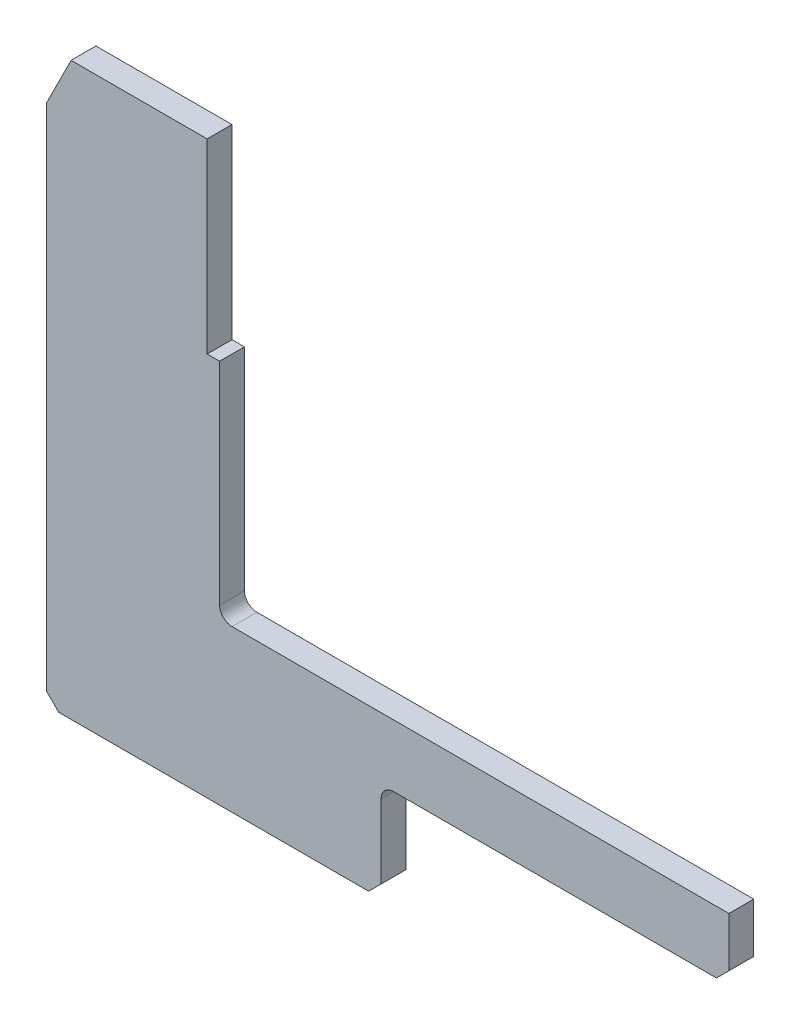
from build123d import *

# Parameters (mm, degrees)
BOSS_EXTRUDE1_DEPTH = 40
CHAMFER1_SIZE       = 20
FILLET1_R           = 20


with BuildPart() as part:
    # Sketch1 → Boss-Extrude1 (new body)
    with BuildSketch(Plane.XY):
        Polygon((-572.578678855, 758.246779508), (-572.578678855, -80.753220492), (-33.578678855, -80.753220492), (-33.578678855, 78.246779508), (526.421321145, 78.246779508), (526.421321145, 178.246779508), (-293.578678855, 178.246779508), (-293.578678855, 538.246779508), (-313.578678855, 538.246779508), (-313.578678855, 838.246779508), (-532.578678855, 838.246779508), align=None)
    extrude(amount=BOSS_EXTRUDE1_DEPTH)

    # Chamfer1
    chamfer1_edges = [part.edges().sort_by_distance(p)[0] for p in [
        (-572.578678855, -80.753220492, 20),
        (526.421321145, 78.246779508, 20),
        (-33.578678855, -80.753220492, 20),
    ]]
    chamfer(chamfer1_edges, length=CHAMFER1_SIZE)

    # Fillet1
    fillet1_edges = [part.edges().sort_by_distance(p)[0] for p in [
        (-293.578678855, 178.246779508, 20),
        (-33.578678855, 78.246779508, 20),
    ]]
    fillet(fillet1_edges, radius=FILLET1_R)


solid = part.part
